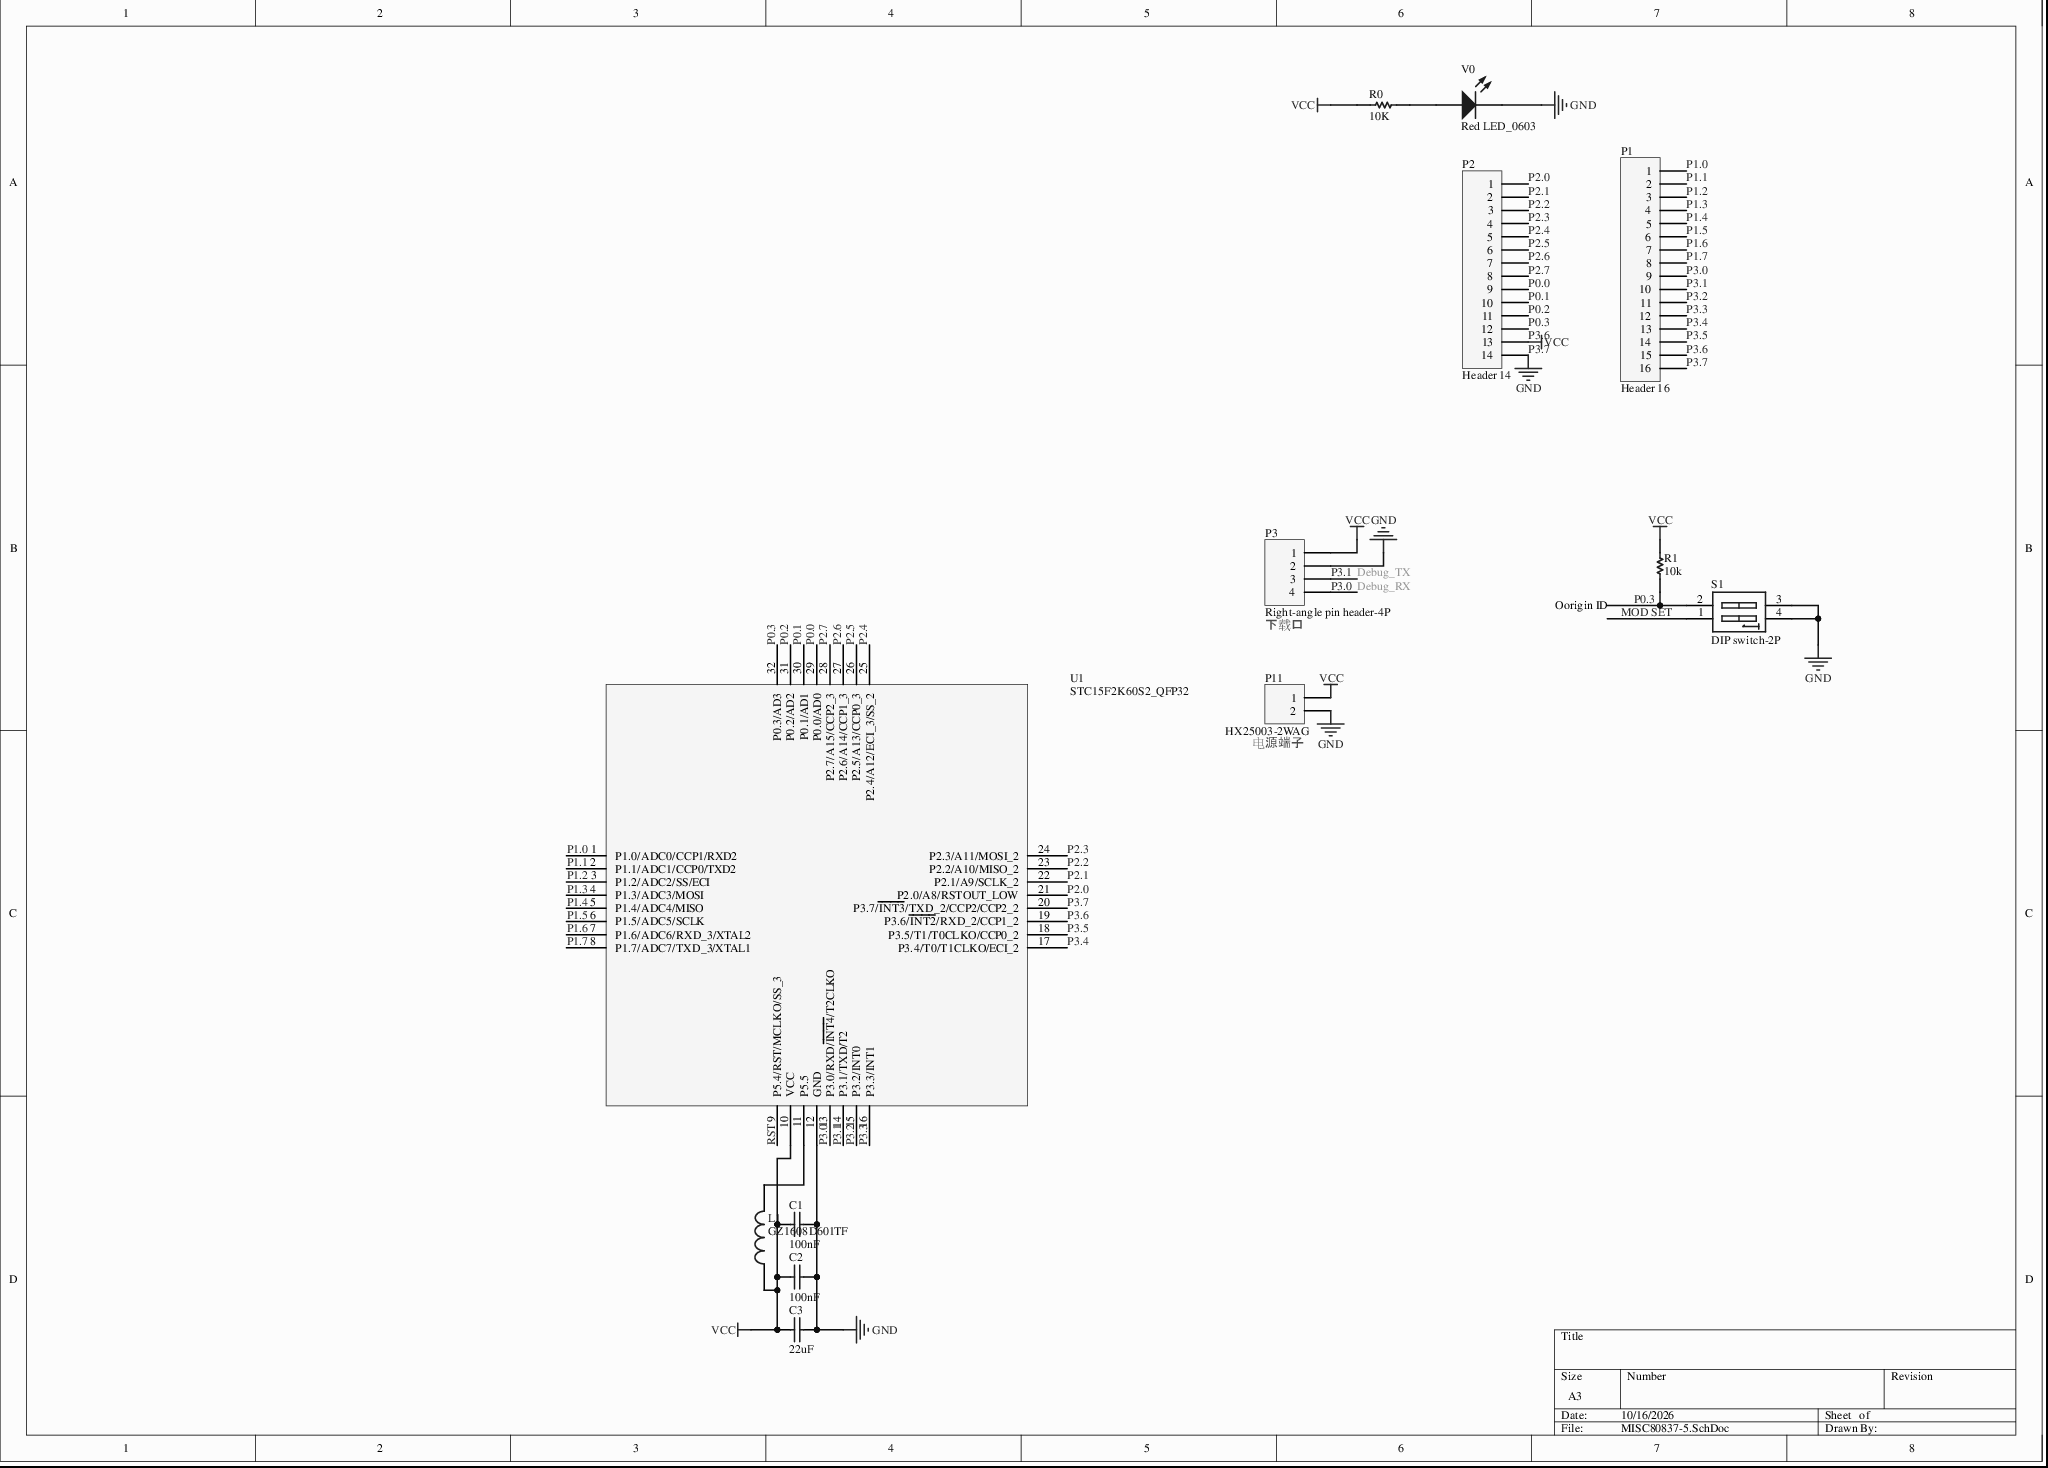
[diagram p0: MISC80837-5.SchDoc]
# Altium project MISC80837-3.PrjPcb
1 sheet, 13 parts. Net scope: global (net labels, ports and power ports of the same name join across sheets).
Board file: MISC80837.PcbDoc

## Sheet MISC80837-5.SchDoc
size A3

### Parts
C1  100nF  [C0603]
C2  100nF  [C0603]
C3  22uF  [C0603]
L1  GZ1608D601TF  [AL0204]
P1  Header 16  [HDR1X16]
P2  Header 14  [HDR1X14]
P3  Right-angle pin header-4P  [HDR1X4]
P11  HX25003-2WAG  [HDR1X2]
R0  10K  [6-0805_N]
R1  10k  [6-0805_N]
S1  DIP switch-2P  [DIP-4]
U1  STC15F2K60S2_QFP32  [LQFP32]
V0  Red LED_0603  [3.2X1.6X1.1]

### Nets
P3.6: C1.2 C2.2 C3.2 L1.1 P1.15 P2.13 P3.1 P11.1 R0.1 R1.2 U1.10(VCC) U1.19(P3.6/~{INT2}/RXD_2/CCP1_2)  [also labelled VCC]
P3.7: C1.1 C2.1 C3.1 P1.16 P2.14 P3.2 P11.2 S1.3(B2) S1.4(B1) U1.12(GND) U1.20(P3.7/~{INT3}/TXD_2/CCP2/CCP2_2) V0.2(K)  [also labelled GND]
Debug_RX: P1.9 P3.4 U1.13(P3.0/RXD/~{INT4}/T2CLKO)  [also labelled P3.0]
Debug_TX: P1.10 P3.3 U1.14(P3.1/TXD/T2)  [also labelled P3.1]
MOD SET: S1.1(A1)
Oorigin ID: P2.12 R1.1 S1.2(A2) U1.32(P0.3/AD3)  [also labelled P0.3]
P0.0: P2.9 U1.29(P0.0/AD0)
P0.1: P2.10 U1.30(P0.1/AD1)
P0.2: P2.11 U1.31(P0.2/AD2)
P1.0: P1.1 U1.1(P1.0/ADC0/CCP1/RXD2)
P1.1: P1.2 U1.2(P1.1/ADC1/CCP0/TXD2)
P1.2: P1.3 U1.3(P1.2/ADC2/SS/ECI)
P1.3: P1.4 U1.4(P1.3/ADC3/MOSI)
P1.4: P1.5 U1.5(P1.4/ADC4/MISO)
P1.5: P1.6 U1.6(P1.5/ADC5/SCLK)
P1.6: P1.7 U1.7(P1.6/ADC6/RXD_3/XTAL2)
P1.7: P1.8 U1.8(P1.7/ADC7/TXD_3/XTAL1)
P2.0: P2.1 U1.21(P2.0/A8/RSTOUT_LOW)
P2.1: P2.2 U1.22(P2.1/A9/SCLK_2)
P2.2: P2.3 U1.23(P2.2/A10/MISO_2)
P2.3: P2.4 U1.24(P2.3/A11/MOSI_2)
P2.4: P2.5 U1.25(P2.4/A12/ECI_3/SS_2)
P2.5: P2.6 U1.26(P2.5/A13/CCP0_3)
P2.6: P2.7 U1.27(P2.6/A14/CCP1_3)
P2.7: P2.8 U1.28(P2.7/A15/CCP2_3)
P3.2: P1.11 U1.15(P3.2/INT0)
P3.3: P1.12 U1.16(P3.3/INT1)
P3.4: P1.13 U1.17(P3.4/T0/T1CLKO/ECI_2)
P3.5: P1.14 U1.18(P3.5/T1/T0CLKO/CCP0_2)
RST: U1.9(P5.4/RST/MCLKO/SS_3)
NetL1_2: L1.2 U1.11(P5.5)
NetR0_2: R0.2 V0.1(A)

### Notes on the sheet
- Labels drawn without touching a wire or pin: 下载口, 电源端子

### Library data of the parts
C1-C3 = CAP: Non-polarized capacitor
L1 = INDUCTOR
P1 = Header 16: Header, 16-Pin; LatestRevisionDate: 17-Jul-2002; LatestRevisionNote: Re-released for DXP Platform.; Publisher: Altium Limited
P2 = Header 14: Header, 14-Pin; LatestRevisionDate: 17-Jul-2002; LatestRevisionNote: Re-released for DXP Platform.; Publisher: Altium Limited
P3 = Header 4: Header, 4-Pin; LatestRevisionDate: 17-Jul-2002; LatestRevisionNote: Re-released for DXP Platform.; Publisher: Altium Limited
P11 = Header 2H: Header, 2-Pin, Right Angle; LatestRevisionDate: 17-Jul-2002; LatestRevisionNote: Re-released for DXP Platform.; Publisher: Altium Limited
R0 R1 = RES
S1 = SW DIP-2: DIP Switch, 2 Position, SPST; Published: 24-Mar-1999; LatestRevisionDate: 17-Jul-2002; LatestRevisionNote: Re-released for DXP Platform.; PackageReference: DIP-4; Publisher: Altium Limited
V0 = LED1: Typical RED GaAs LED; Published: 8-Jun-2000; LatestRevisionDate: 08-Jul-2005; LatestRevisionNote: Mech Layer 1 removed.; PackageReference: LED-1; PackageDescription: LED; 2 Leads; Publisher: Altium Limited